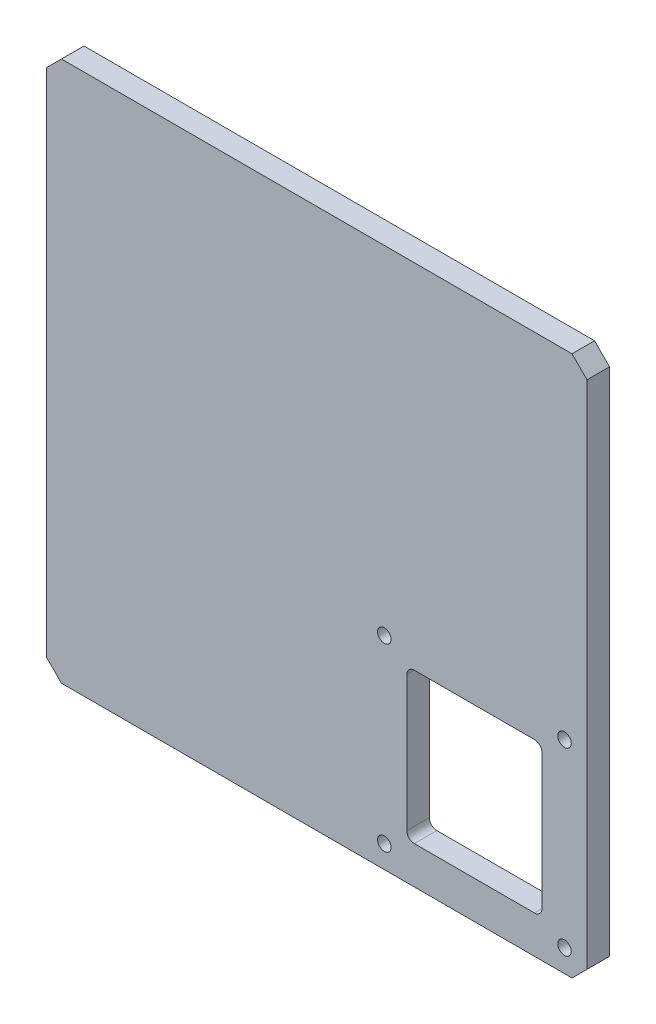
from build123d import *

# Parameters (mm, degrees)
SKETCH1_W                    = 360
SKETCH1_H                    = 360
BOSS_EXTRUDE1_DEPTH          = 15
CHAMFER1_SIZE                = 10
F_9_0_9_DIAMETER_HOLE1_D     = 9
F_9_0_9_DIAMETER_HOLE1_DEPTH = 19.75
F_9_0_9_DIAMETER_HOLE1_TIP   = 2.703872786
SKETCH5_W                    = 90
SKETCH5_H                    = 100
CUT_EXTRUDE2_DEPTH           = 15
FILLET1_R                    = 5


with BuildPart() as part:
    # Sketch1 → Boss-Extrude1 (new body)
    with BuildSketch(Plane.XY):
        Rectangle(SKETCH1_W, SKETCH1_H)
    extrude(amount=BOSS_EXTRUDE1_DEPTH)

    # Chamfer1
    chamfer1_edges = [part.edges().sort_by_distance(p)[0] for p in [
        (-180, 180, 7.5),
        (180, 180, 7.5),
        (180, -180, 7.5),
        (-180, -180, 7.5),
    ]]
    chamfer(chamfer1_edges, length=CHAMFER1_SIZE)

    # Ø9.0 (9) Diameter Hole1
    with Locations(Plane.XY.offset(15)):
        with Locations((165, -45), (45, -45), (45, -165), (165, -165)):
            Hole(F_9_0_9_DIAMETER_HOLE1_D / 2, depth=F_9_0_9_DIAMETER_HOLE1_DEPTH)
            with Locations((0, 0, -(F_9_0_9_DIAMETER_HOLE1_DEPTH + F_9_0_9_DIAMETER_HOLE1_TIP / 2))):  # 118° drill point
                Cone(0, F_9_0_9_DIAMETER_HOLE1_D / 2, F_9_0_9_DIAMETER_HOLE1_TIP, mode=Mode.SUBTRACT)

    # Sketch5 → Cut-Extrude2 (cut)
    with BuildSketch(Plane.XY.offset(15)):
        with Locations((105, -105)):
            Rectangle(SKETCH5_W, SKETCH5_H)
    extrude(amount=-CUT_EXTRUDE2_DEPTH, mode=Mode.SUBTRACT)

    # Fillet1
    fillet1_edges = [part.edges().sort_by_distance(p)[0] for p in [
        (150, -55, 7.5),
        (150, -155, 7.5),
        (60, -155, 7.5),
        (60, -55, 7.5),
    ]]
    fillet(fillet1_edges, radius=FILLET1_R)


solid = part.part
